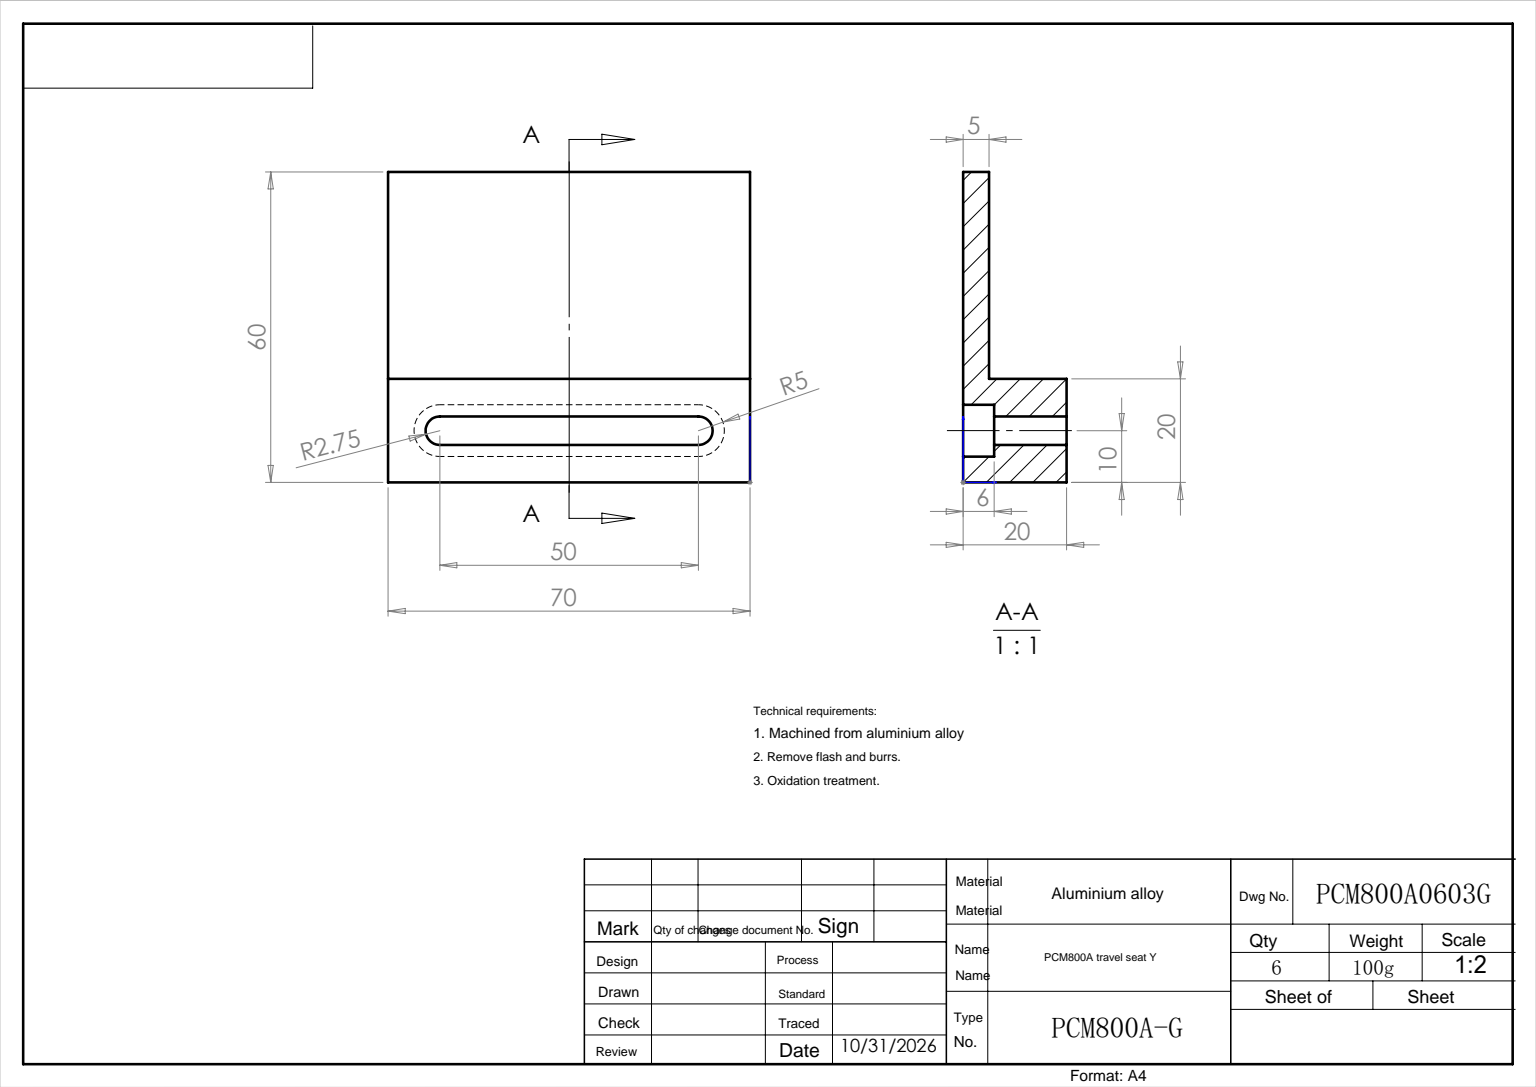
SolidWorks part; units mm, degrees
ref_plane "前视基准面" through (0, 0, 0) normal (0, 0, 1) x (1, 0, 0)
ref_plane "上视基准面" through (0, 0, 0) normal (0, 1, 0) x (1, 0, 0)
ref_plane "右视基准面" through (0, 0, 0) normal (1, 0, 0) x (0, 0, -1)
sketch "草图1" plane through (0, 0, 0) normal (0, 0, 1) x (1, 0, 0)
  line L0 (0, 0) -> (0, 60)
  line L1 (0, 60) -> (5, 60)
  line L2 (5, 60) -> (5, 20)
  line L3 (5, 20) -> (20, 20)
  line L4 (20, 20) -> (20, 0)
  line L5 (20, 0) -> (0, 0)
  dimension "D1" = 5
  dimension "D2" = 15
  dimension "D3" = 40
  dimension "D4" = 60
extrude "凸台-拉伸1" add sketch "草图1" along normal blind 70
sketch "草图3" plane through (0, 0, 0) normal (-1, 0, 0) x (0, 0, 1)
  line L0 (-4.2966, 10) -> (127.9844, 10) construction
  line L1 (70, 20) -> (0, 20) construction
  line L3 (10, 12.75) -> (60, 12.75)
  line L4 (10, 7.25) -> (60, 7.25)
  line L5 (0, 60) -> (0, 0) construction
  line L6 (70, 60) -> (70, 0) construction
  arc A0 (10, 12.75) -> (10, 7.25) centre (10, 10) ccw
  arc A1 (60, 7.25) -> (60, 12.75) centre (60, 10) ccw
  dimension "D2" = 5.5
  dimension "D3" = 5.5
  dimension "D4" = 10
  dimension "D5" = 10
  dimension "D1" = 10
extrude "切除-拉伸1" cut sketch "草图3" against normal blind 1200
sketch "草图6" plane through (0, 0, 0) normal (-1, 0, 0) x (0, 0, 1)
  line L6 (10, 5) -> (60, 5)
  line L7 (60, 15) -> (10, 15)
  line L8 (10, 5) -> (60, 5)
  line L9 (60, 15) -> (10, 15)
  arc A8 (60, 5) -> (60, 15) centre (60, 10) ccw
  arc A9 (10, 15) -> (10, 5) centre (10, 10) ccw
  arc A10 (60, 5) -> (60, 15) centre (60, 10) ccw
  arc A11 (10, 15) -> (10, 5) centre (10, 10) ccw
  dimension "D1" = 2.25
extrude "切除-拉伸2" cut sketch "草图6" against normal blind 6
